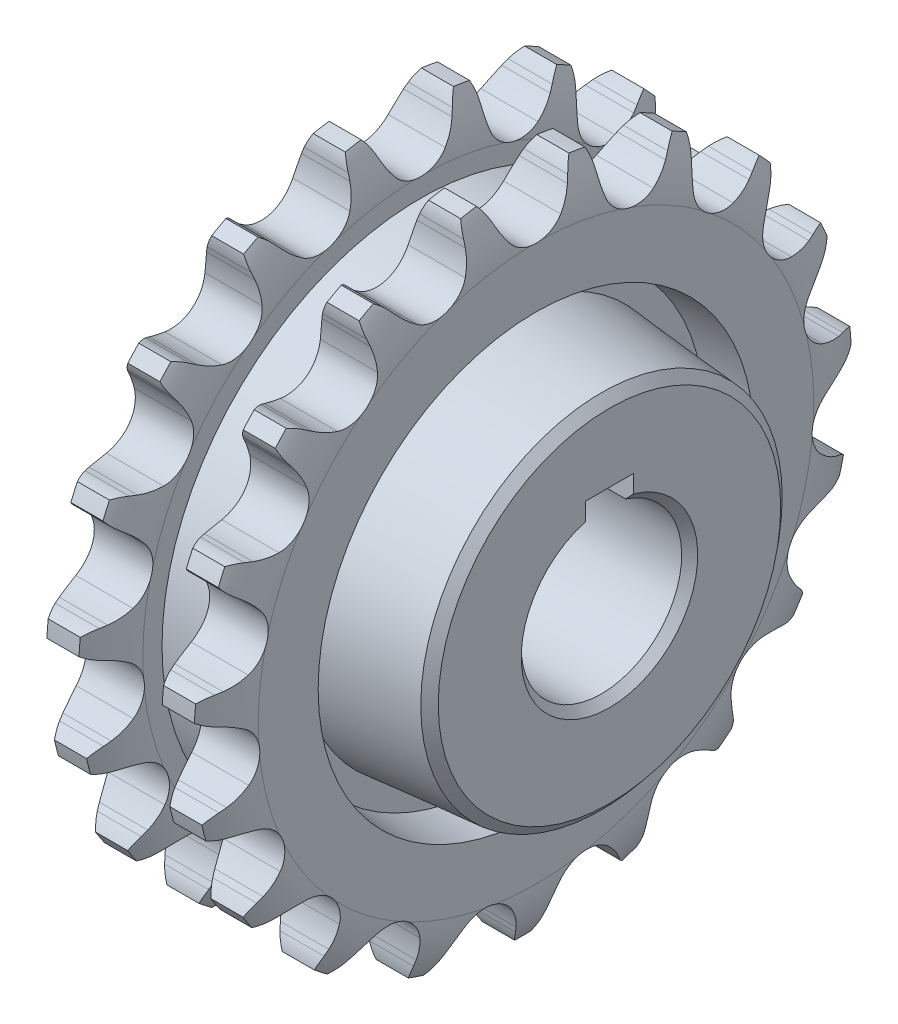
SolidWorks part; units mm, degrees
material "AISI 304"
ref_plane "Front Plane" through (0, 0, 0) normal (0, 0, 1) x (1, 0, 0)
ref_plane "Top Plane" through (0, 0, 0) normal (0, 1, 0) x (1, 0, 0)
ref_plane "Right Plane" through (0, 0, 0) normal (1, 0, 0) x (0, 0, -1)
sketch "Sketch1" plane through (0, 0, 0) normal (0, 0, 1) x (1, 0, 0)
  line L0 (-6.35, 0) -> (6.35, 0) construction
  line L1 (-5.15, 10) -> (-5.15, 27.1496) construction
  line L2 (-5.15, 27.1496) -> (-3.6503, 27.1496) construction
  line L3 (-3.6503, 27.1496) -> (-3.6503, 34.6196)
  line L4 (-1.9993, 41) -> (1.9993, 41)
  line L5 (3.6503, 34.6196) -> (3.6503, 27.1496)
  line L6 (3.6503, 27.1496) -> (5.15, 27.1496) construction
  line L7 (5.15, 27.1496) -> (5.15, 10) construction
  line L8 (5.15, 10) -> (-5.15, 10) construction
  line L9 (0, 0) -> (0, 41) construction
  line L10 (-3.0556, 38.5796) -> (3.0556, 38.5796) construction
  line L11 (-3.0556, -38.5796) -> (3.0556, -38.5796) construction
  line L12 (6.35, 0) -> (25.35, 0) construction
  line L13 (-3.6503, 34.6196) -> (3.6503, 34.6196) construction
  line L14 (-3.6503, -34.6196) -> (3.6503, -34.6196) construction
  line L15 (25.35, 0) -> (33.27, 0) construction
  line L16 (33.27, 0) -> (45.34, 0) construction
  line L17 (45.34, 0) -> (53.19, 0) construction
  line L18 (53.19, 0) -> (67.57, 0) construction
  line L19 (-3.6503, 32.2296) -> (3.6503, 32.2296) construction
  line L20 (-5.15, 27.1496) -> (5.15, 27.1496) construction
  line L21 (-3.6503, 27.1496) -> (3.6503, 27.1496)
  arc A0 (-1.9993, 41) -> (-3.6503, 34.6196) centre (9.0492, 34.7373) ccw
  arc A1 (1.9993, 41) -> (3.6503, 34.6196) centre (-9.0492, 34.7373) cw
  point P30 (3.6503, 27.1496)
  point P33 (-3.6503, 27.1496)
  dimension "rx" = 12.7
  dimension "d" = 77.1593
  dimension "p" = 12.7
  dimension "z" = 19
  dimension "da" = 82
  dimension "df" = 69.2393
  dimension "dr" = 7.92
  dimension "dk" = 20
  dimension "h" = 12.07
  dimension "bf1" = 7.3005
  dimension "b1" = 7.85
  dimension "ba" = 1.651
  dimension "pt" = 14.38
  dimension "t" = 10.3
  dimension "C2" = 11.43
  dimension "c1" = 6.35
revolve "Revolve1" add sketch "Sketch1" angle 360 about L0
sketch "Sketch2" plane through (0, 0, 0) normal (1, 0, 0) x (0, 0, -1)
  line L0 (0, 0) -> (0, 41) construction
  line L1 (0, 0) -> (-6.7484, 40.4408) construction
  line L2 (0, 0) -> (-13.3127, 38.7785) construction
  line L3 (3.1687, 36.0899) -> (-0.6147, 39.0627) construction
  line L4 (4.5522, 38.4265) -> (-4.9821, 42.4942) construction
  line L5 (0, 0) -> (6.7484, 40.4408) construction
  line L6 (4.5522, 38.4265) -> (4.8587, 39.1448)
  line L7 (-4.5522, 38.4265) -> (-4.8587, 39.1448)
  circle A0 centre (0, 0) radius 41 construction
  arc A1 (3.1687, 36.0899) -> (-3.1687, 36.0899) centre (0, 38.5796) cw
  arc A2 (3.1687, 36.0899) -> (4.5522, 38.4265) centre (-4.9821, 42.4942) ccw
  arc A3 (5.7509, 40.5947) -> (4.8587, 39.1448) centre (10.1556, 36.885) ccw
  arc A4 (-3.1687, 36.0899) -> (-4.5522, 38.4265) centre (4.9821, 42.4942) cw
  arc A5 (-5.7509, 40.5947) -> (-4.8587, 39.1448) centre (-10.1556, 36.885) cw
  arc A7 (5.7509, 40.5947) -> (-5.7509, 40.5947) centre (0, 0) ccw
  dimension "r1" = 4.0298
  dimension "r3" = 5.7588
  dimension "D1" = 18.947
  dimension "D2" = 9.474
  dimension "α/2" = 51.842
  dimension "M" = 4.9821
  dimension "T" = 3.9146
  dimension "β" = 15.053
  dimension "γ/2" = 13.632
  dimension "bc" = 0.781
extrude "Cut-Extrude1" cut sketch "Sketch2" against normal mid plane 10.9508
pattern_circular "CirPattern1" count 19 over 360 about axis through (0, 0, 0) along (1, 0, 0) of "Cut-Extrude1"
pattern_linear "LPattern1" count 2 spacing 14.38 along (1, 0, 0) of bodies 103
sketch "Sketch5" plane through (0, 0, 0) normal (0, 0, 1) x (1, 0, 0)
  line L0 (7.19, 10) -> (7.19, 23.7375) construction
  line L1 (-12.81, 10) -> (27.19, 10)
  line L2 (-12.81, 10) -> (-12.81, 22.4383)
  line L3 (-12.81, 22.4383) -> (2.04, 23.7375)
  line L4 (27.19, 10) -> (27.19, 22.4383)
  line L5 (-3.6503, 27.1496) -> (-3.6503, 34.6196) construction
  line L6 (7.19, 23.7375) -> (7.19, 169.716) construction
  line L7 (0, 0) -> (-10.4728, 0) construction
  line L9 (2.04, 23.7375) -> (12.34, 23.7375) construction
  line L11 (12.34, 23.7375) -> (27.19, 22.4383)
  line L12 (3.6503, 32.2296) -> (10.7297, 32.2296)
  line L13 (12.34, 26.6518) -> (12.34, 23.7375)
  line L14 (-3.6503, 27.1496) -> (2.04, 26.6518)
  line L15 (2.04, 26.6518) -> (2.04, 23.7375)
  line L16 (3.6503, 32.2296) -> (-3.6503, 27.1496)
  line L17 (-5.15, 27.1496) -> (5.15, 27.1496) construction
  line L18 (18.0302, 27.1496) -> (12.34, 26.6518)
  line L19 (10.7297, 32.2296) -> (18.0302, 27.1496)
  point P26 (7.19, 32.2296)
  dimension "D1" = 5
  dimension "L" = 40
  dimension "H" = 12.4383
  dimension "D2" = 10.8403
  dimension "D3" = 5
  dimension "D4" = 10.3
revolve "Revolve2" add sketch "Sketch5" angle 360 about L7
sketch "Sketch4" plane through (-12.81, 0, 0) normal (-1, 0, 0) x (0, 0, 1)
  line L1 (-3, 9.5394) -> (3, 9.5394)
  line L2 (-3, 9.5394) -> (-3, 12.8)
  line L3 (-3, 12.8) -> (3, 12.8)
  line L4 (3, 9.5394) -> (3, 12.8)
  circle A1 centre (0, 0) radius 10 construction
  point P4 (0, 12.8)
  dimension "D1" = 22.8
  dimension "键槽宽度" = 6
  dimension "t1" = 3
chamfer "Chamfer1" distance 1 angle 45 4 edges at (27.19, 0, -10) (27.19, 0, -22.4383) (-12.81, 0, -10) (-12.81, 0, -22.4383)
extrude "Cut-Extrude4" cut sketch "Sketch4" against normal through all
ref_plane "Plane1" through (14.38, 0, 0) normal (1, 0, 0) x (0, 0, -1)
